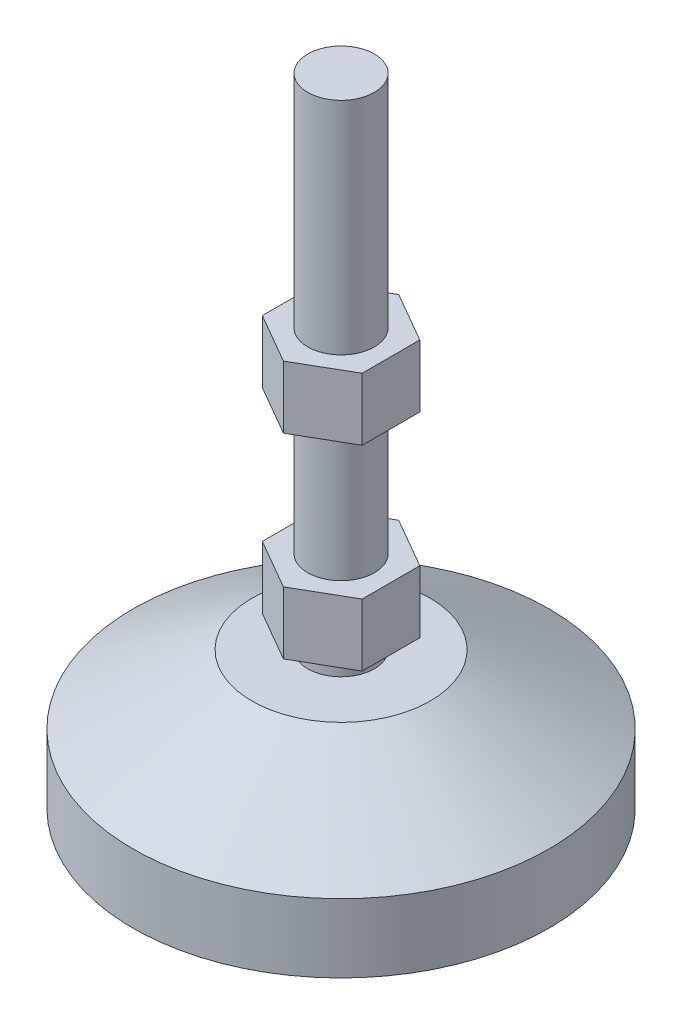
SolidWorks part; units mm, degrees
material "厂家标准"
ref_plane "前视基准面" through (0, 0, 0) normal (0, 0, 1) x (1, 0, 0)
ref_plane "上视基准面" through (0, 0, 0) normal (0, 1, 0) x (1, 0, 0)
ref_plane "右视基准面" through (0, 0, 0) normal (1, 0, 0) x (0, 0, -1)
sketch "草图1" plane through (0, 0, 0) normal (0, 0, 1) x (1, 0, 0)
  line L0 (0, 0) -> (50, 0)
  line L1 (50, 0) -> (50, 16.5)
  line L2 (50, 16.5) -> (21.4212, 33)
  line L3 (21.4212, 33) -> (0, 33)
  line L4 (0, 0) -> (0, 33) construction
  line L5 (0, 33) -> (0, 0)
revolve "旋转1" add sketch "草图1" angle 360 about L4
sketch "草图2" plane through (0, 33, 0) normal (0, 1, 0) x (1, 0, 0)
  line L1 (12, -6.9282) -> (12, 6.9282)
  line L2 (12, 6.9282) -> (0, 13.8564)
  line L3 (0, 13.8564) -> (-12, 6.9282)
  line L4 (-12, 6.9282) -> (-12, -6.9282)
  line L5 (-12, -6.9282) -> (0, -13.8564)
  line L6 (0, -13.8564) -> (12, -6.9282)
  circle A0 centre (0, 0) radius 12 construction
  dimension "螺母宽度" = 24
extrude "凸台-拉伸1" add sketch "草图2" along normal blind 15 from offset 5
sketch "草图3" plane through (0, 53, 0) normal (0, 1, 0) x (1, 0, 0)
  circle A0 centre (0, 0) radius 8
  dimension "螺杆直径" = 16
extrude "凸台-拉伸2" add sketch "草图3" along normal blind 100 and the other way up to surface (53 mm away)
cosmetic thread "装饰螺纹线1" parameters "D2"=0.1
sketch "草图4" plane through (0, 0, 0) normal (0, 1, 0) x (1, 0, 0)
  line L12 (0, -13.8564) -> (12, -6.9282)
  line L13 (12, -6.9282) -> (12, 6.9282)
  line L14 (12, 6.9282) -> (0, 13.8564)
  line L15 (0, 13.8564) -> (-12, 6.9282)
  line L16 (-12, 6.9282) -> (-12, -6.9282)
  line L17 (-12, -6.9282) -> (0, -13.8564)
  line L18 (0, -13.8564) -> (12, -6.9282)
  line L19 (12, -6.9282) -> (12, 6.9282)
  line L20 (12, 6.9282) -> (0, 13.8564)
  line L21 (0, 13.8564) -> (-12, 6.9282)
  line L22 (-12, 6.9282) -> (-12, -6.9282)
  line L23 (-12, -6.9282) -> (0, -13.8564)
  dimension "D1" = 0
extrude "凸台-拉伸3" add sketch "草图4" against normal blind 15 from offset 100
equation "\"D1@草图1\"=\"底盘高度@草图1\"/2"
equation "\"D1@凸台-拉伸3\"=\"螺母厚@凸台-拉伸1\""
equation "\"底盘高度@草图1\"=int(\"底盘直径@草图1\"/3)"
